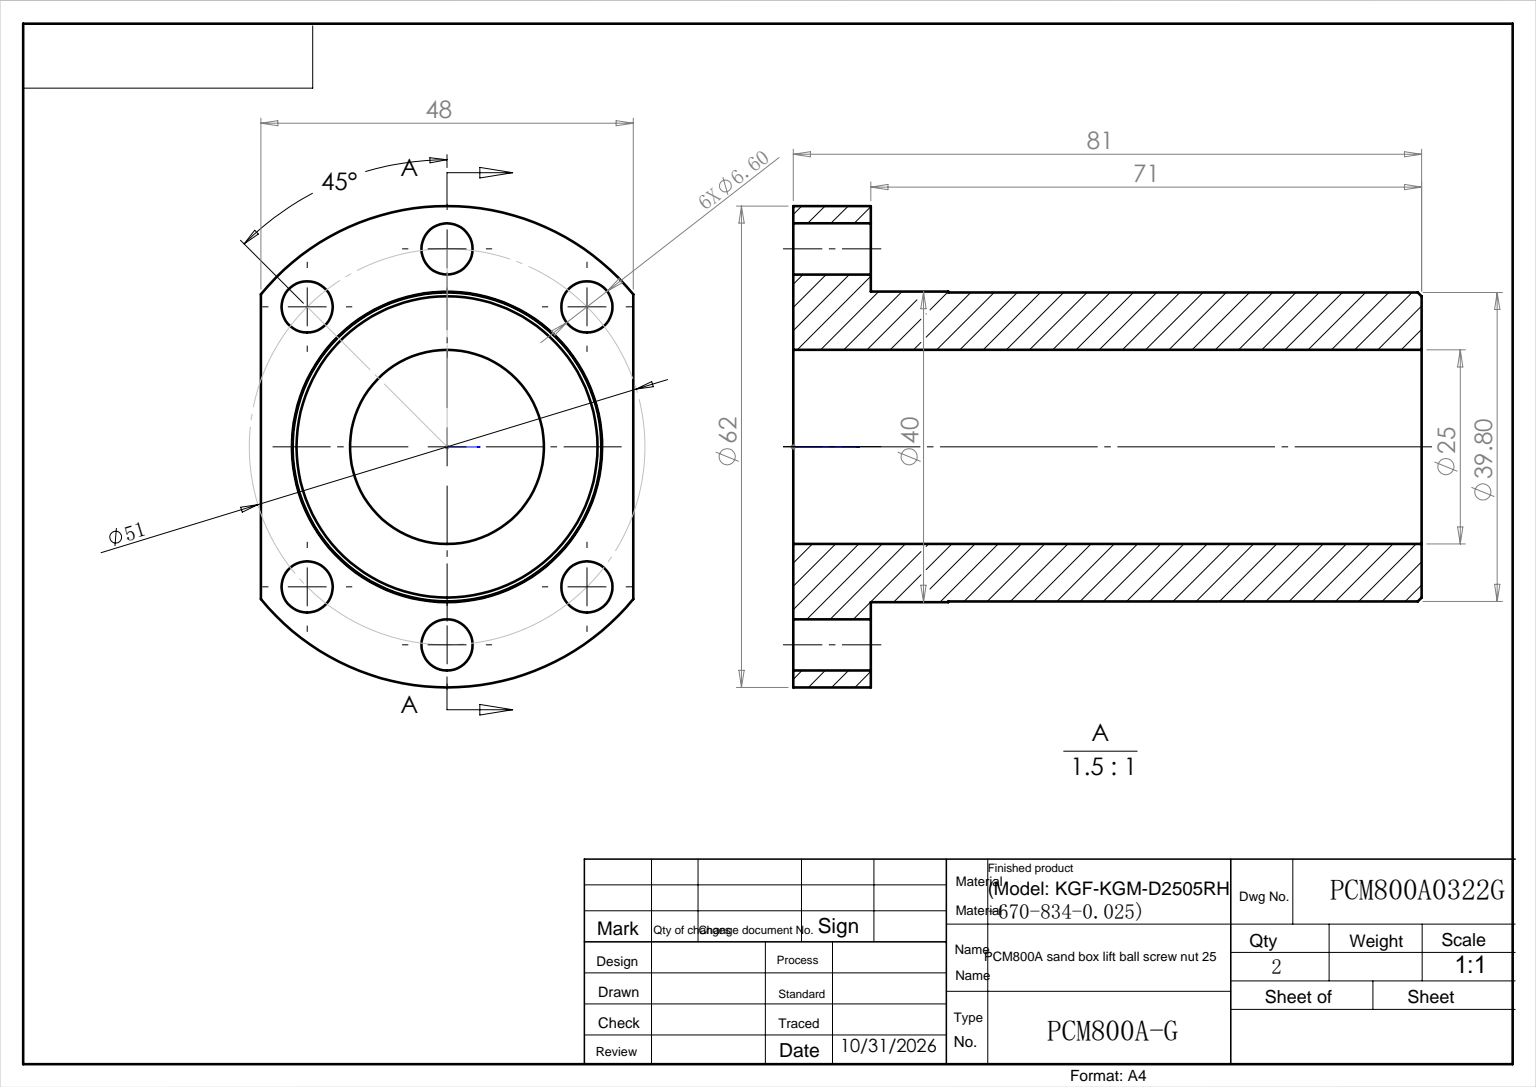
SolidWorks part; units mm, degrees
ref_plane "前视基准面" through (0, 0, 0) normal (0, 0, 1) x (1, 0, 0)
ref_plane "上视基准面" through (0, 0, 0) normal (0, 1, 0) x (1, 0, 0)
ref_plane "右视基准面" through (0, 0, 0) normal (1, 0, 0) x (0, 0, -1)
sketch "草图1" plane through (0, 0, 0) normal (0, 1, 0) x (1, 0, 0)
  line L2 (24, -19.5954) -> (24, 19.6475)
  line L3 (-24, -19.5954) -> (-24, 19.6475)
  arc A0 (-24, -19.5954) -> (24, -19.5954) centre (0, 0.0261) ccw
  arc A2 (24, 19.6475) -> (-24, 19.6475) centre (0, 0.0261) ccw
  dimension "D1" = 48
  dimension "D2" = 24
extrude "拉伸1" add sketch "草图1" along normal blind 10
sketch "草图2" plane through (0, 10, 0) normal (0, 1, 0) x (-1, 0, 0)
  circle A0 centre (0, 0) radius 20
extrude "拉伸2" add sketch "草图2" along normal blind 10
sketch "草图3" plane through (0, 20, 0) normal (0, 1, 0) x (-1, 0, 0)
  circle A0 centre (0, 0) radius 19.9
extrude "拉伸3" add sketch "草图3" along normal blind 61
sketch "草图5" plane through (0, 81, 0) normal (0, 1, 0) x (-1, 0, 0)
  circle A0 centre (0, 0) radius 12.5
extrude "切除-拉伸1" cut sketch "草图5" against normal through all
sketch "草图6" plane through (0, 0, 0) normal (0, -1, 0) x (1, 0, 0)
  circle A0 centre (0, 0) radius 25.5 construction
  circle A2 centre (18.0312, -18.0312) radius 3.3
  circle A3 centre (0, -25.5) radius 3.3
  circle A4 centre (-18.0312, -18.0312) radius 3.3
  circle A6 centre (-18.0312, 18.0312) radius 3.3
  circle A7 centre (0, 25.5) radius 3.3
  circle A8 centre (18.0312, 18.0312) radius 3.3
  circle A11 centre (25.5, 0) radius 3.3
  circle A12 centre (-25.5, 0) radius 3.3
extrude "切除-拉伸2" cut sketch "草图6" against normal through all
chamfer "倒角1" distance 0.5 angle 45 1 edges at (0, 81, 19.9)
